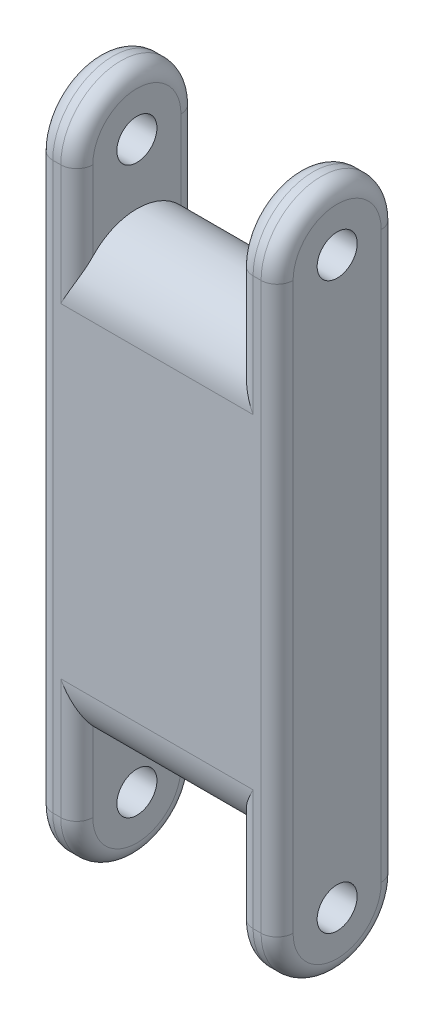
from build123d import *

# Parameters (mm, degrees)
BOSS_EXTRUDE1_DEPTH = 19.05
SKETCH2_R           = 1.5875
SKETCH2_R_2         = 1.5874999999999988
CUT_EXTRUDE1_DEPTH  = 19.05
CUT_EXTRUDE2_DEPTH  = 6.35
FILLET1_R           = 1.27
SKETCH3_R           = 1.3523393116529026
BOSS_EXTRUDE2_DEPTH = 2.54
FILLET2_R           = 0.762
SKETCH4_R           = 0.6365323226185287
CUT_EXTRUDE3_DEPTH  = 50.150613196033525
SCALE_RATIO_1_SCALE = 1.3


with BuildPart() as part:
    # Sketch1 → Boss-Extrude1 (new body)
    with BuildSketch(Plane(origin=(0, 0, 0), x_dir=(0, 0, -1), z_dir=(1, 0, 0))):
        with BuildLine():
            Line((-4.7625, 0), (-4.7625, 44.8056))
            ThreePointArc((-4.7625, 44.8056), (2.9e-16, 49.5681), (4.7625, 44.8056))
            Line((4.7625, 44.8056), (4.762500000000005, 5.8e-16))
            ThreePointArc((4.762500000000005, 5.8e-16), (1.35e-15, -4.762500000000005), (-4.7625, 0))
        make_face()
    extrude(amount=BOSS_EXTRUDE1_DEPTH)

    # Sketch2 → Cut-Extrude1 (cut)
    with BuildSketch(Plane(origin=(19.05, 0, 0), x_dir=(0, 0, -1), z_dir=(1, 0, 0))):
        Circle(SKETCH2_R)
        with Locations((0, 44.8056)):
            Circle(SKETCH2_R_2)
    extrude(amount=-CUT_EXTRUDE1_DEPTH, mode=Mode.SUBTRACT)

    # 3DSketch1 → Cut-Extrude2 (cut, symmetric)
    with BuildSketch(Plane(origin=(9.524999999999954, 44.80559999999997, -4.762500000000004), x_dir=(0, -0.9781419365644765, 0.20793833685469326), z_dir=(-1, -9.3e-16, 3.6e-16))):
        with BuildLine():
            Line((0, 0), (9.316801945776646, -1.9806126585409503))
            ThreePointArc((9.316801945776646, -1.9806126585409503), (5.6487073021588, 3.668094643617845), (11.2974146043176, 7.336189287235693))
            Line((11.2974146043176, 7.336189287235693), (1.9806126585409412, 9.316801945776648))
            ThreePointArc((1.9806126585409412, 9.316801945776648), (-3.6680946436178474, 5.648707302158794), (0, 0))
        make_face()
        with BuildLine():
            Line((45.806849011474235, 0), (36.49004706569759, 1.980612658540955))
            ThreePointArc((36.49004706569759, 1.980612658540955), (40.15814170931544, -3.668094643617836), (34.50943440715664, -7.336189287235687))
            Line((34.50943440715664, -7.336189287235687), (43.82623635293327, -9.316801945776637))
            ThreePointArc((43.82623635293327, -9.316801945776637), (49.47494365509206, -5.648707302158793), (45.806849011474235, 0))
        make_face()
    extrude(amount=CUT_EXTRUDE2_DEPTH, both=True, mode=Mode.SUBTRACT)

    # Fillet1
    fillet1_edges = [part.edges().sort_by_distance(p)[0] for p in [
        (19.05, 49.5681, 7e-17),
        (19.05, 22.4028, 4.7625),
        (15.874999999999961, 40.04309999999998, 4.762500000000003),
        (15.874999999999957, 40.043099999999974, -4.762500000000005),
        (3.174999999999959, 40.04309999999996, -4.762499999999999),
        (3.1749999999999625, 40.04309999999997, 4.762500000000008),
        (19.05, -4.762500000000005, -2.98e-15),
        (0, 22.4028, 4.7625),
        (0, 49.5681, 7e-17),
        (15.874999999999995, 4.762500000000003, 4.762499999999996),
        (15.874999999999991, 4.762500000000003, -4.762500000000006),
        (3.1749999999999954, 4.762499999999989, 4.762500000000001),
        (3.174999999999992, 4.762499999999989, -4.762500000000001),
        (0, 22.4028, -4.762500000000003),
        (0, -4.762500000000005, -2.98e-15),
        (19.05, 22.4028, -4.762500000000003),
    ]]
    fillet(fillet1_edges, radius=FILLET1_R)

    # Sketch3 → Boss-Extrude2 (add)
    with BuildSketch(Plane.ZY):
        with Locations((-2.068463746823568, 42.49092897757123)):
            Circle(SKETCH3_R)
    extrude(amount=BOSS_EXTRUDE2_DEPTH)

    # Fillet2
    fillet2_edges = [part.edges().sort_by_distance(p)[0] for p in [
        (-2.54, 42.49092897757123, -3.42080305847647),
    ]]
    fillet(fillet2_edges, radius=FILLET2_R)

    # Sketch4 → Cut-Extrude3 (cut, through all)
    with BuildSketch(Plane(origin=(0, 10.403230824440865, 18.01892435079848), x_dir=(-1, 0, 0), z_dir=(0, 0.49999999999999484, 0.8660254037844416))):
        with Locations(Location((0.8782218587697344, -37.93359892462922, 0), (0, 0, 90))):
            Circle(SKETCH4_R)
    extrude(amount=-CUT_EXTRUDE3_DEPTH, mode=Mode.SUBTRACT)


with BuildPart() as part_1:
    # Scale ratio 1: scaled about (0, 0, 0)
    add(part.part.scale(SCALE_RATIO_1_SCALE))


solid = part_1.part
